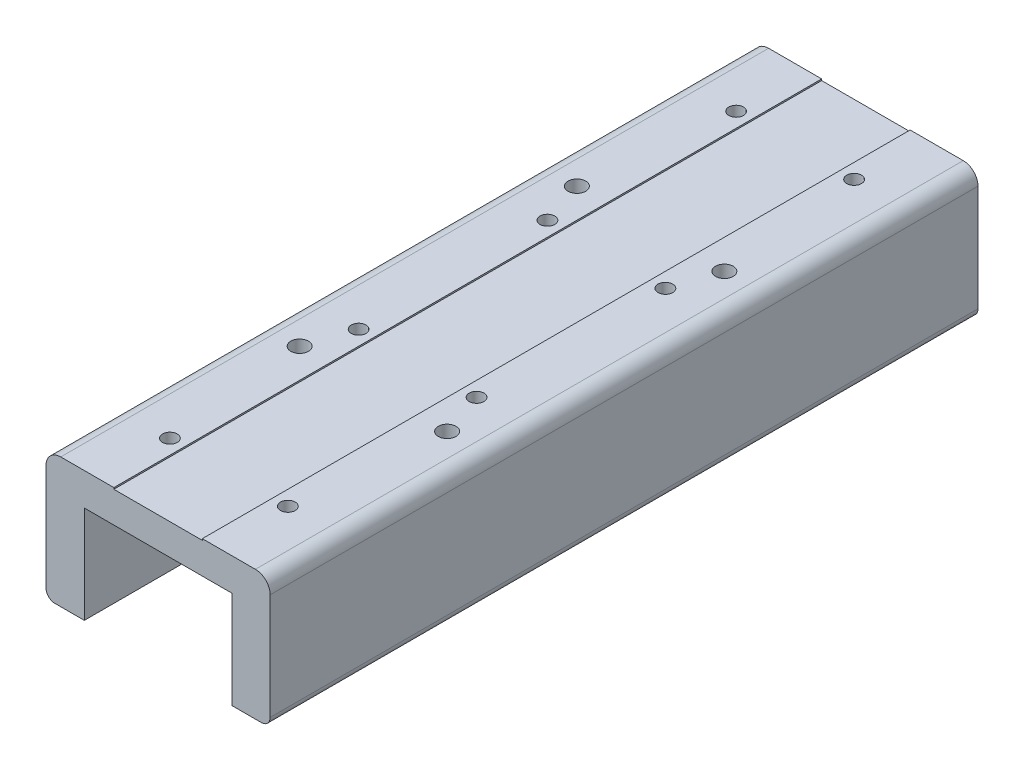
from build123d import *

# Parameters (mm, degrees)
EXTRUDE_406_DEPTH   = 240
SKETCH_3_R          = 2.5
SKETCH_3_R_2        = 3
CUT_EXTRUDE_1_DEPTH = 10


with BuildPart() as part:
    # 草图1 → Extrude 406 (new body)
    with BuildSketch(Plane.XY):
        with BuildLine():
            Line((33, 50.785428571), (15, 50.785428571))
            Line((15, 50.785428571), (15, 50.285428571))
            Line((15, 50.285428571), (-15, 50.285428571))
            Line((-15, 50.285428571), (-15, 50.785428571))
            Line((-15, 50.785428571), (-33, 50.785428571))
            ThreePointArc((-33, 50.785428571), (-36.535533906, 49.320962477), (-38, 45.785428571))
            Line((-38, 45.785428571), (-38, 9.785428571))
            ThreePointArc((-38, 9.785428571), (-37.121320344, 7.664108228), (-35, 6.785428571))
            Line((-35, 6.785428571), (-25, 6.785428571))
            Line((-25, 6.785428571), (-25, 39.785428571))
            Line((-25, 39.785428571), (25, 39.785428571))
            Line((25, 39.785428571), (25, 6.785428571))
            Line((25, 6.785428571), (35, 6.785428571))
            ThreePointArc((35, 6.785428571), (37.121320344, 7.664108228), (38, 9.785428571))
            Line((38, 9.785428571), (38, 45.785428571))
            ThreePointArc((38, 45.785428571), (36.535533906, 49.320962477), (33, 50.785428571))
        make_face()
    extrude(amount=-EXTRUDE_406_DEPTH)

    # 草图3 → 切除-拉伸1 (cut)
    with BuildSketch(Plane(origin=(0, 50.785428571, 0), x_dir=(-1, 0, 0), z_dir=(0, 1, 0))):
        with Locations((-20, -24)):
            Circle(SKETCH_3_R)
        with Locations((20, -24)):
            Circle(SKETCH_3_R)
        with Locations((-20, -88)):
            Circle(SKETCH_3_R)
        with Locations((20, -88)):
            Circle(SKETCH_3_R)
        with Locations((-20, -152)):
            Circle(SKETCH_3_R)
        with Locations((20, -152)):
            Circle(SKETCH_3_R)
        with Locations((-20, -216)):
            Circle(SKETCH_3_R)
        with Locations((20, -216)):
            Circle(SKETCH_3_R)
        with Locations((-25, -73)):
            Circle(SKETCH_3_R_2)
        with Locations((25, -73)):
            Circle(SKETCH_3_R_2)
        with Locations((-25, -167)):
            Circle(SKETCH_3_R_2)
        with Locations((25, -167)):
            Circle(SKETCH_3_R_2)
    extrude(amount=-CUT_EXTRUDE_1_DEPTH, mode=Mode.SUBTRACT)


solid = part.part
